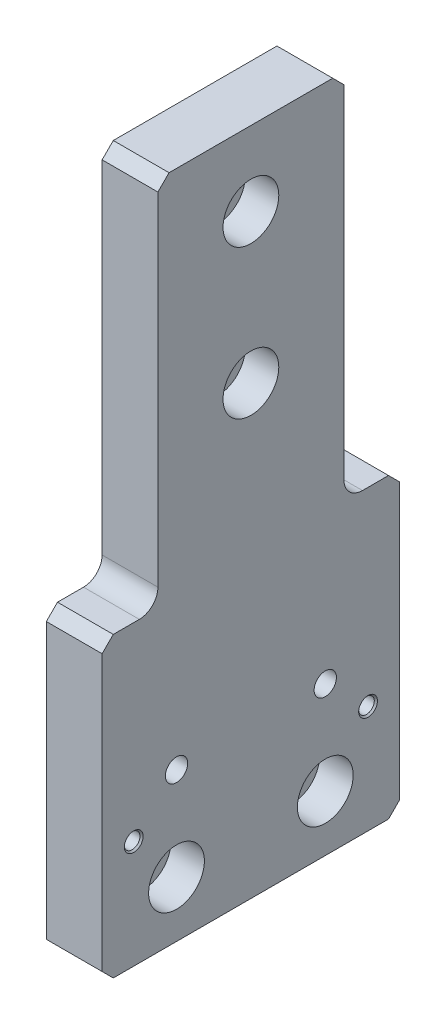
SolidWorks part; units mm, degrees
material "45#"
ref_plane "Front Plane" through (0, 0, 0) normal (0, 0, 1) x (1, 0, 0)
ref_plane "Top Plane" through (0, 0, 0) normal (0, 1, 0) x (1, 0, 0)
ref_plane "Right Plane" through (0, 0, 0) normal (1, 0, 0) x (0, 0, -1)
sketch "Sketch1" plane through (0, 0, 0) normal (1, 0, 0) x (0, 0, -1)
  line L0 (0, 0) -> (0, 180) construction
  line L5 (40, 0) -> (-40, 0)
  line L6 (-40, 0) -> (-40, 80)
  line L7 (-40, 80) -> (-25, 80)
  line L8 (-25, 80) -> (-25, 180)
  line L9 (-25, 180) -> (25, 180)
  line L10 (25, 80) -> (25, 180)
  line L11 (40, 80) -> (25, 80)
  line L12 (40, 0) -> (40, 80)
  point P11 (0, 180)
  dimension "D1" = 50
  dimension "D2" = 180
  dimension "D3" = 100
  dimension "D4" = 80
extrude "Boss-Extrude1" add sketch "Sketch1" along normal blind 15
hole_wizard "M5 Tapped Hole1" positions "Sketch2" profile "Sketch3" tap size "M5" standard "GB"
sketch "Sketch2" plane through (15, 0, 0) normal (1, 0, 0) x (0, 0, -1)
  point P0 (31.5, 29)
  point P3 (-31.5, 29)
sketch "Sketch3" plane through (15, 29, -31.5) normal (0, 1, 0) x (0, 0, -1)
  line L0 (0, 0) -> (0, 13.6618)
  line L1 (0, 13.6618) -> (2.1, 12.4)
  line L2 (2.1, 12.4) -> (2.1, 0.425)
  line L3 (2.1, 0.425) -> (2.525, 0)
  line L5 (2.525, 0) -> (0, 0)
  line L6 (-2.1, 0.425) -> (-2.525, 0) construction
  line L10 (0, 13.6618) -> (-2.1, 12.4) construction
  line L11 (0, -6.35) -> (0, 107.95) construction
  dimension "螺纹孔钻头直径" = 4.2
  dimension "螺纹孔钻头深度" = 12.4
  dimension "近端锥形沉头孔直径" = 5.05
  dimension "近端锥形沉头孔角度" = 90
  dimension "导头角度" = 118
cosmetic thread "Cosmetic thread 1" parameters "D1"=10, "D2"=5
cosmetic thread "Cosmetic thread 2" parameters "D1"=10, "D2"=5
hole_wizard "CBORE for M8 Hexagon socket head cap screws1" positions "Sketch4" profile "Sketch5" counterbore size "M8" standard "GB" end condition through all
sketch "Sketch4" plane through (15, 0, 0) normal (1, 0, 0) x (0, 0, -1)
  line L0 (0, 0) -> (0, 180) construction
  line L1 (25, 180) -> (-25, 180) construction
  point P0 (0, 160)
  point P2 (0, 120)
  dimension "D1" = 40
  dimension "D2" = 20
sketch "Sketch5" plane through (15, 160, 0) normal (0, 1, 0) x (0, 0, -1)
  line L0 (0, 0) -> (0, 15)
  line L1 (0, 15) -> (4.5, 15)
  line L3 (4.5, 15) -> (4.5, 9)
  line L4 (4.5, 9) -> (7.5, 9)
  line L5 (7.5, 9) -> (7.5, 0)
  line L7 (7.5, 0) -> (0, 0)
  line L11 (0, -6.35) -> (0, 107.95) construction
  dimension "通孔孔直径" = 9
  dimension "通孔孔深度" = 15
  dimension "柱形沉头孔直径" = 15
  dimension "柱形沉头孔深度" = 9
hole_wizard "CBORE for M8 Hexagon socket head cap screws2" positions "Sketch6" profile "Sketch7" counterbore size "M8" standard "GB" end condition through all
sketch "Sketch6" plane through (15, 0, 0) normal (1, 0, 0) x (0, 0, -1)
  line L0 (-40, 0) -> (40, 0) construction
  line L1 (0, 0) -> (0, 180) construction
  line L2 (25, 180) -> (-25, 180) construction
  point P0 (-20, 15)
  point P2 (20, 15)
  dimension "D1" = 40
  dimension "D2" = 15
sketch "Sketch7" plane through (15, 15, 20) normal (0, 1, 0) x (0, 0, -1)
  line L0 (0, 0) -> (0, 15)
  line L1 (0, 15) -> (4.5, 15)
  line L3 (4.5, 15) -> (4.5, 9)
  line L4 (4.5, 9) -> (7.5, 9)
  line L5 (7.5, 9) -> (7.5, 0)
  line L7 (7.5, 0) -> (0, 0)
  line L11 (0, -6.35) -> (0, 107.95) construction
  dimension "通孔孔直径" = 9
  dimension "通孔孔深度" = 15
  dimension "柱形沉头孔直径" = 15
  dimension "柱形沉头孔深度" = 9
hole_wizard "Ø6.0mm blind hole 1" positions "Sketch8" profile "Sketch9" hole size "Ø6.0" standard "GB" end condition through all
sketch "Sketch8" plane through (15, 0, 0) normal (1, 0, 0) x (0, 0, -1)
  line L0 (0, 0) -> (0, 180) construction
  line L1 (25, 180) -> (-25, 180) construction
  circle A0 centre (20, 15) radius 4.5 construction
  point P0 (-20, 40)
  point P2 (20, 40)
  dimension "D1" = 40
  dimension "D2" = 25
sketch "Sketch9" plane through (15, 40, 20) normal (0, 1, 0) x (0, 0, -1)
  line L0 (0, 0) -> (0, 15)
  line L1 (0, 15) -> (3, 15)
  line L2 (3, 15) -> (3, 0)
  line L5 (3, 0) -> (0, 0)
  line L11 (0, -6.35) -> (0, 107.95) construction
  dimension "通孔孔直径" = 6
  dimension "通孔孔深度" = 15
fillet "Fillet1" radius 5 2 edges at (7.5, 80, -25) (7.5, 80, 25)
chamfer "Chamfer1" distance 3 angle 45 6 edges at (7.5, 180, -25) (7.5, 80, -40) (7.5, 0, -40) (7.5, 0, 40) (7.5, 80, 40) (7.5, 180, 25)
